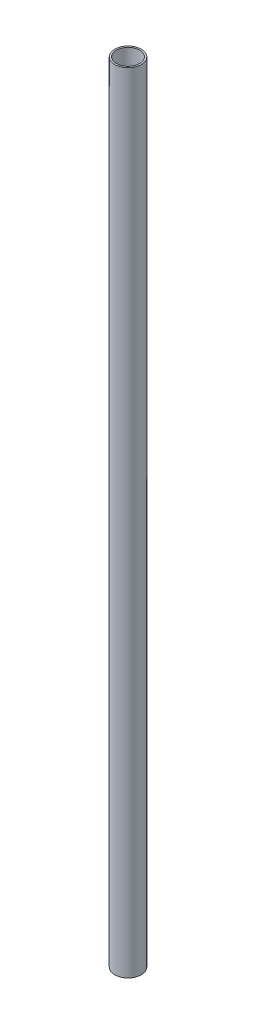
SolidWorks part; units mm, degrees
material "Thornel Mat VMA"
ref_plane "前视基准面" through (0, 0, 0) normal (0, 0, 1) x (1, 0, 0)
ref_plane "上视基准面" through (0, 0, 0) normal (0, 1, 0) x (1, 0, 0)
ref_plane "右视基准面" through (0, 0, 0) normal (1, 0, 0) x (0, 0, -1)
other "Configuration Table"
sketch "草图1" plane through (0, 0, 0) normal (0, 1, 0) x (1, 0, 0)
  circle A0 centre (0, 0) radius 8
  dimension "D1" = 16
extrude "拉伸-薄壁1" add sketch "草图1" along normal blind 475 thin thin type one direction reverse wall 1
